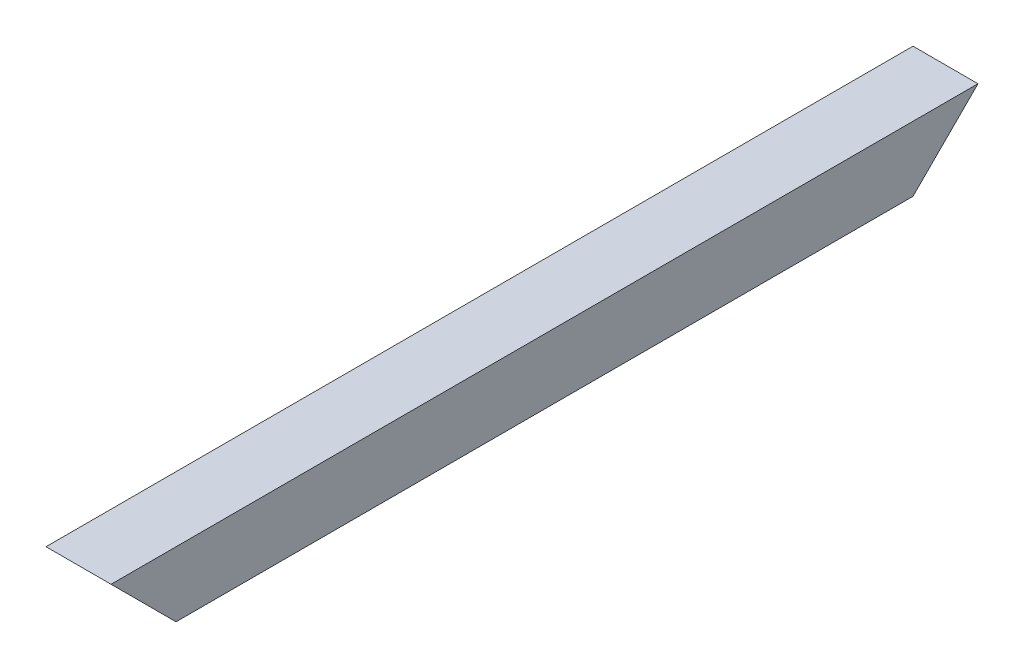
from build123d import *

# Parameters (mm, degrees)
SKETCH1_W           = 30
SKETCH1_H           = 30
BOSS_EXTRUDE1_DEPTH = 400
SKETCH2_W           = 24
SKETCH2_H           = 24
CUT_EXTRUDE1_DEPTH  = 492
CUT_EXTRUDE3_DEPTH  = 402.958781438
CUT_EXTRUDE6_DEPTH  = 402.958781438


with BuildPart() as part:
    # Sketch1 → Boss-Extrude1 (new body)
    with BuildSketch(Plane.XY):
        with Locations((-30.141748722, 10.901003365)):
            Rectangle(SKETCH1_W, SKETCH1_H)
    extrude(amount=BOSS_EXTRUDE1_DEPTH)

    # Sketch2 → Cut-Extrude1 (cut)
    with BuildSketch(Plane.XY.offset(400)):
        with Locations((-30.141748722, 10.901003365)):
            Rectangle(SKETCH2_W, SKETCH2_H)
    extrude(amount=-CUT_EXTRUDE1_DEPTH, mode=Mode.SUBTRACT)

    # Sketch4 → Cut-Extrude3 (cut, through all)
    with BuildSketch(Plane(origin=(-15.141748722, 0, 0), x_dir=(0, 0, -1), z_dir=(1, 0, 0))):
        Polygon((0, 25.901003365), (-30, -4.098996635), (0, -4.098996635), align=None)
    extrude(amount=-CUT_EXTRUDE3_DEPTH, mode=Mode.SUBTRACT)

    # Sketch8 → Cut-Extrude6 (cut, through all)
    with BuildSketch(Plane(origin=(-15.141748722, 0, 0), x_dir=(0, 0, -1), z_dir=(1, 0, 0))):
        Polygon((-400, 25.901003365), (-370, -4.098996635), (-400, -4.098996635), align=None)
    extrude(amount=-CUT_EXTRUDE6_DEPTH, mode=Mode.SUBTRACT)


solid = part.part
